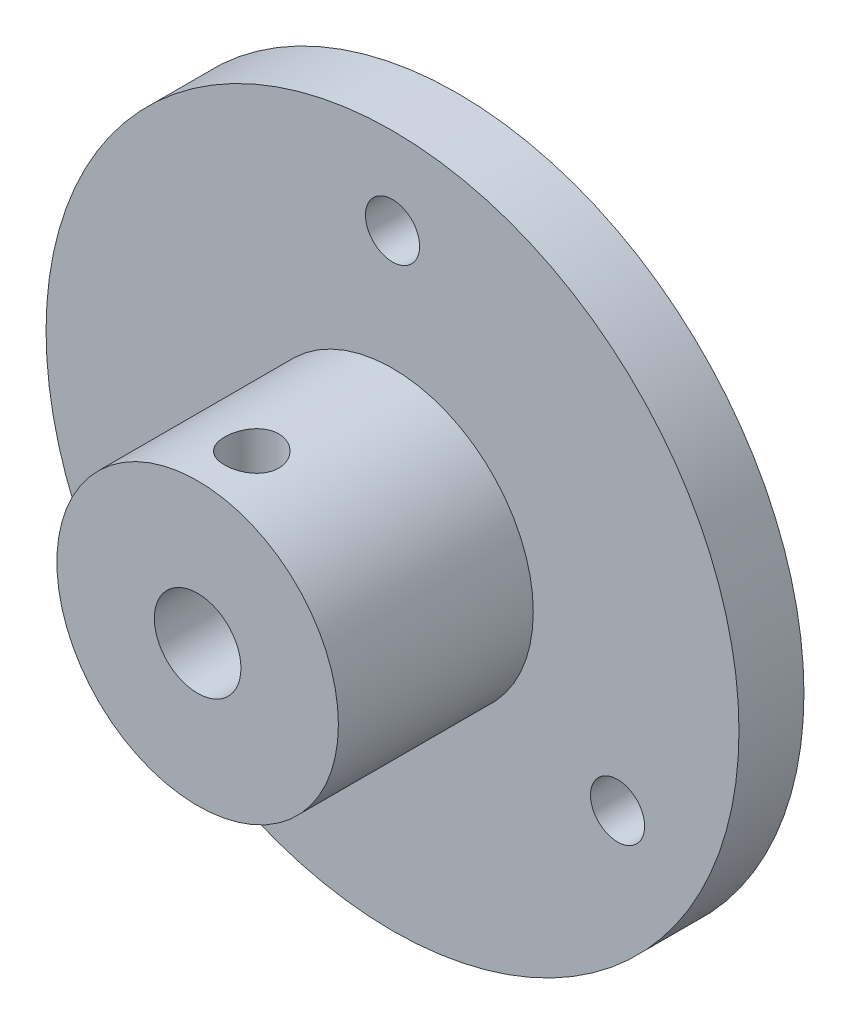
SolidWorks part; units mm, degrees
ref_plane "Front Plane" through (0, 0, 0) normal (0, 0, 1) x (1, 0, 0)
ref_plane "Top Plane" through (0, 0, 0) normal (0, 1, 0) x (1, 0, 0)
ref_plane "Right Plane" through (0, 0, 0) normal (1, 0, 0) x (0, 0, -1)
sketch "Sketch1" plane through (0, 0, 0) normal (0, 0, 1) x (1, 0, 0)
  circle A0 centre (0, 0) radius 16
  dimension "D1" = 32
extrude "Boss-Extrude1" add sketch "Sketch1" along normal blind 3
sketch "Sketch2" plane through (0, 0, 3) normal (0, 0, 1) x (1, 0, 0)
  circle A0 centre (0, 0) radius 6.5
  point P3 (2.0519, -22.134)
  dimension "D1" = 13
extrude "Boss-Extrude2" add sketch "Sketch2" along normal blind 9
sketch "Sketch3" plane through (0, 0, 0) normal (0, 0, -1) x (-1, 0, 0)
  circle A0 centre (0, 0) radius 2
  dimension "D1" = 4
extrude "Cut-Extrude1" cut sketch "Sketch3" against normal blind 22
sketch "Sketch4" plane through (0, 0, 0) normal (0, 0, -1) x (-1, 0, 0)
  circle A0 centre (0, 12) radius 1
  circle A1 centre (10.3923, -6) radius 1
  circle A2 centre (-10.3923, -6) radius 1
  point P9 (0, 0)
  dimension "D2" = 2
  dimension "D1" = 12
  dimension "D3" = 3
sketch "Sketch13" plane through (0, 0, 0) normal (0, 1, 0) x (1, 0, 0)
  line L0 (-6.5, -12) -> (6.5, -12) construction
  point P0 (0, -9.5)
  dimension "D1" = 2.5
hole_wizard "M3 Tapped Hole5" positions "Sketch15" profile "Sketch16" tap size "M3" standard "GB"
sketch "Sketch15" plane through (0, 0, 0) normal (0, 1, 0) x (1, 0, 0)
  point P0 (0, -9.5)
sketch "Sketch16" plane through (0, 0, 9.5) normal (1, 0, 0) x (0, 0, -1)
  line L0 (0, 0) -> (0, 8.2511)
  line L1 (0, 8.2511) -> (1.25, 7.5)
  line L2 (1.25, 7.5) -> (1.25, 0)
  line L5 (1.25, 0) -> (0, 0)
  line L10 (0, 8.2511) -> (-1.25, 7.5) construction
  line L11 (0, -6.35) -> (0, 107.95) construction
  dimension "螺纹孔钻头直径" = 2.5
  dimension "螺纹孔钻头深度" = 7.5
  dimension "导头角度" = 118
cosmetic thread "CosmeticThread21" parameters "D1"=6, "D2"=3
extrude "Cut-Extrude2" cut sketch "Sketch4" against normal blind 10
hole_wizard "M3 Tapped Hole6" positions "Sketch17" profile "Sketch18" tap size "M3" standard "GB" end condition up to next
sketch "Sketch17" plane through (0, 0, 0) normal (0, 0, -1) x (-1, 0, 0)
  point P0 (0, 12)
  point P3 (-10.3923, -6)
  point P6 (10.3923, -6)
sketch "Sketch18" plane through (0, 12, 0) normal (1, 0, 0) x (0, 1, 0)
  line L0 (0, 0) -> (0, 12)
  line L1 (0, 12) -> (1.25, 12)
  line L2 (1.25, 12) -> (1.25, 0)
  line L5 (1.25, 0) -> (0, 0)
  line L11 (0, -6.35) -> (0, 107.95) construction
  dimension "通孔螺纹孔钻头直径" = 2.5
  dimension "通孔螺纹孔钻头深度" = 12
cosmetic thread "CosmeticThread22" parameters "D2"=3
cosmetic thread "CosmeticThread23" parameters "D2"=3
cosmetic thread "CosmeticThread24" parameters "D2"=3
